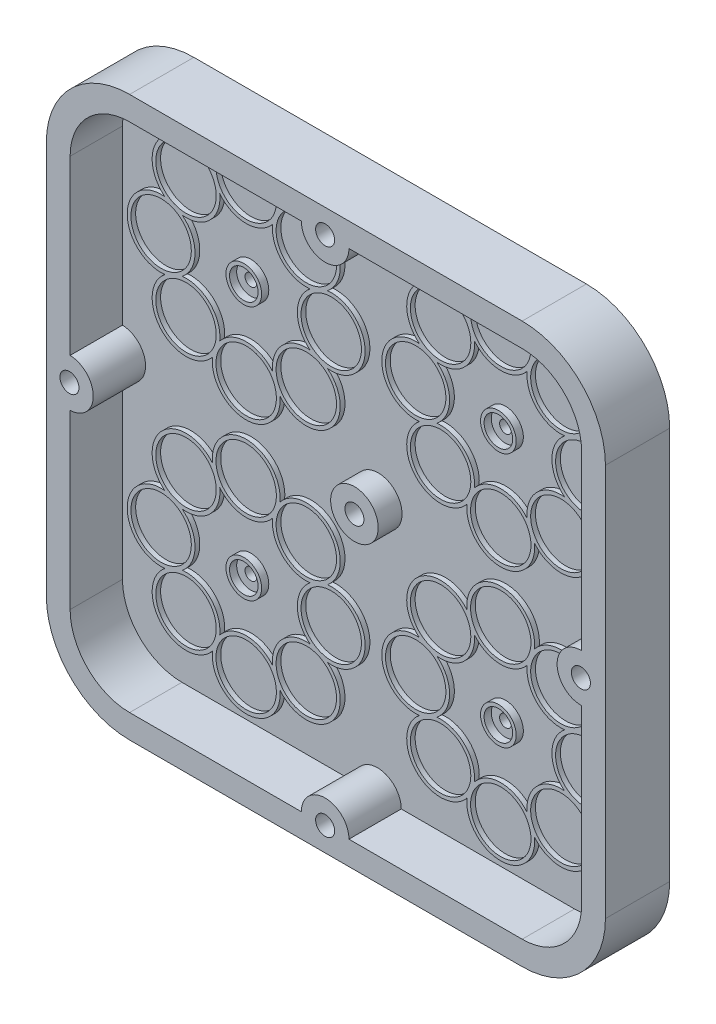
from build123d import *

# Parameters (mm, degrees)
SKETCH1_R           = 4
SKETCH1_R_2         = 2.5
BOSS_EXTRUDE1_DEPTH = 5
SKETCH2_R           = 4
BOSS_EXTRUDE2_DEPTH = 22
SKETCH3_R           = 10
SKETCH3_R_2         = 4
BOSS_EXTRUDE3_DEPTH = 10
SKETCH4_R           = 12.7
BOSS_EXTRUDE4_DEPTH = 2
SKETCH5_R           = 7.5
SKETCH5_R_2         = 6
BOSS_EXTRUDE5_DEPTH = 3


with BuildPart() as part:
    # Sketch1 → Boss-Extrude1 (new body)
    with BuildSketch(Plane.XY):
        with BuildLine():
            Line((35, 0), (200, 0))
            ThreePointArc((200, 0), (224.748737342, 10.251262658), (235, 35))
            Line((235, 35), (235, 200))
            ThreePointArc((235, 200), (224.748737342, 224.748737342), (200, 235))
            Line((200, 235), (35, 235))
            ThreePointArc((35, 235), (10.251262658, 224.748737342), (0, 200))
            Line((0, 200), (0, 35))
            ThreePointArc((0, 35), (10.251262658, 10.251262658), (35, 0))
        make_face()
        with Locations((117.5, 225)):
            Circle(SKETCH1_R, mode=Mode.SUBTRACT)
        with Locations((117.5, 10)):
            Circle(SKETCH1_R, mode=Mode.SUBTRACT)
        with Locations((117.5, 117.5)):
            Circle(SKETCH1_R, mode=Mode.SUBTRACT)
        with Locations((225, 117.5)):
            Circle(SKETCH1_R, mode=Mode.SUBTRACT)
        with Locations((10, 117.5)):
            Circle(SKETCH1_R, mode=Mode.SUBTRACT)
        with Locations((64, 171)):
            Circle(SKETCH1_R_2, mode=Mode.SUBTRACT)
        with Locations((171, 171)):
            Circle(SKETCH1_R_2, mode=Mode.SUBTRACT)
        with Locations((171, 64)):
            Circle(SKETCH1_R_2, mode=Mode.SUBTRACT)
        with Locations((64, 64)):
            Circle(SKETCH1_R_2, mode=Mode.SUBTRACT)
    extrude(amount=BOSS_EXTRUDE1_DEPTH)

    # Sketch2 → Boss-Extrude2 (add)
    with BuildSketch(Plane.XY.offset(5)):
        with BuildLine():
            Line((235, 35), (235, 200))
            ThreePointArc((235, 200), (224.748737342, 224.748737342), (200, 235))
            Line((200, 235), (35, 235))
            ThreePointArc((35, 235), (10.251262658, 224.748737342), (0, 200))
            Line((0, 200), (0, 35))
            ThreePointArc((0, 35), (10.251262658, 10.251262658), (35, 0))
            Line((35, 0), (200, 0))
            ThreePointArc((200, 0), (224.748737342, 10.251262658), (235, 35))
        make_face()
        with Locations(Location((117.185983795, 225.007361775, 0), (0, 0, 270.907179338))):
            Circle(SKETCH2_R, mode=Mode.SUBTRACT)
        with Locations(Location((224.685983795, 117.507361775, 0), (0, 0, 270.907179338))):
            Circle(SKETCH2_R, mode=Mode.SUBTRACT)
        with Locations(Location((117.185983795, 10.007361775, 0), (0, 0, 270.907179338))):
            Circle(SKETCH2_R, mode=Mode.SUBTRACT)
        with Locations(Location((9.72235037, 117.506509199, 0), (0, 0, 270.64647273))):
            Circle(SKETCH2_R, mode=Mode.SUBTRACT)
        with BuildLine():
            Line((200, 225), (127.185981085, 225))
            ThreePointArc((127.185981085, 225), (117.185983795, 215.007361775), (107.185986504, 225))
            Line((107.185986504, 225), (35, 225))
            ThreePointArc((35, 225), (17.32233047, 217.67766953), (10, 200))
            Line((10, 200), (10, 127.50265399))
            ThreePointArc((10, 127.50265399), (19.72235037, 117.506509199), (10, 107.510364408))
            Line((10, 107.510364408), (10, 35))
            ThreePointArc((10, 35), (17.32233047, 17.32233047), (35, 10))
            Line((35, 10), (107.185986504, 10))
            ThreePointArc((107.185986504, 10), (117.185983795, 20.007361775), (127.185981085, 10))
            Line((127.185981085, 10), (200, 10))
            ThreePointArc((200, 10), (217.67766953, 17.32233047), (225, 35))
            Line((225, 35), (225, 107.5122933))
            ThreePointArc((225, 107.5122933), (214.685983795, 117.507361775), (225, 127.50243025))
            Line((225, 127.50243025), (225, 200))
            ThreePointArc((225, 200), (217.67766953, 217.67766953), (200, 225))
        make_face(mode=Mode.SUBTRACT)
    extrude(amount=BOSS_EXTRUDE2_DEPTH)

    # Sketch3 → Boss-Extrude3 (add)
    with BuildSketch(Plane.XY.offset(5)):
        with Locations((117.5, 117.5)):
            Circle(SKETCH3_R)
        with Locations((117.5, 117.5)):
            Circle(SKETCH3_R_2, mode=Mode.SUBTRACT)
    extrude(amount=BOSS_EXTRUDE3_DEPTH)

    # Sketch4 → Boss-Extrude4 (add)
    # profile 1 of 4: a face of its own
    with BuildSketch(Plane.XY.offset(5)):
        with BuildLine():
            ThreePointArc((136.802142668, 185.165216311), (121, 171), (136.802142668, 156.834783689))
            ThreePointArc((136.802142668, 156.834783689), (135.644660941, 135.644660941), (156.834783689, 136.802142668))
            ThreePointArc((156.834783689, 136.802142668), (171, 121), (185.165216311, 136.802142668))
            ThreePointArc((185.165216311, 136.802142668), (206.355339059, 135.644660941), (205.197857332, 156.834783689))
            ThreePointArc((205.197857332, 156.834783689), (221, 171), (205.197857332, 185.165216311))
            ThreePointArc((205.197857332, 185.165216311), (206.355339059, 206.355339059), (185.165216311, 205.197857332))
            ThreePointArc((185.165216311, 205.197857332), (171, 221), (156.834783689, 205.197857332))
            ThreePointArc((156.834783689, 205.197857332), (135.644660941, 206.355339059), (136.802142668, 185.165216311))
        make_face()
        with Locations((171, 206.75)):
            Circle(SKETCH4_R, mode=Mode.SUBTRACT)
        with Locations((145.720932573, 196.279067427)):
            Circle(SKETCH4_R, mode=Mode.SUBTRACT)
        with Locations((135.25, 171)):
            Circle(SKETCH4_R, mode=Mode.SUBTRACT)
        with Locations((145.720932573, 145.720932573)):
            Circle(SKETCH4_R, mode=Mode.SUBTRACT)
        with Locations((171, 135.25)):
            Circle(SKETCH4_R, mode=Mode.SUBTRACT)
        with Locations((196.279067427, 145.720932573)):
            Circle(SKETCH4_R, mode=Mode.SUBTRACT)
        with Locations((206.75, 171)):
            Circle(SKETCH4_R, mode=Mode.SUBTRACT)
        with Locations((196.279067427, 196.279067427)):
            Circle(SKETCH4_R, mode=Mode.SUBTRACT)
        with BuildLine():
            ThreePointArc((159.886148884, 197.831210095), (171, 192.5), (182.113851116, 197.831210095))
            ThreePointArc((182.113851116, 197.831210095), (186.202795796, 186.202795796), (197.831210095, 182.113851116))
            ThreePointArc((197.831210095, 182.113851116), (192.5, 171), (197.831210095, 159.886148884))
            ThreePointArc((197.831210095, 159.886148884), (186.202795796, 155.797204204), (182.113851116, 144.168789905))
            ThreePointArc((182.113851116, 144.168789905), (171, 149.5), (159.886148884, 144.168789905))
            ThreePointArc((159.886148884, 144.168789905), (155.797204204, 155.797204204), (144.168789905, 159.886148884))
            ThreePointArc((144.168789905, 159.886148884), (149.5, 171), (144.168789905, 182.113851116))
            ThreePointArc((144.168789905, 182.113851116), (155.797204204, 186.202795796), (159.886148884, 197.831210095))
        make_face(mode=Mode.SUBTRACT)
    # profile 2 of 4: a face of its own
    with BuildSketch(Plane.XY.offset(5)):
        with BuildLine():
            ThreePointArc((185.165216311, 98.197857332), (171, 114), (156.834783689, 98.197857332))
            ThreePointArc((156.834783689, 98.197857332), (135.644660941, 99.355339059), (136.802142668, 78.165216311))
            ThreePointArc((136.802142668, 78.165216311), (121, 64), (136.802142668, 49.834783689))
            ThreePointArc((136.802142668, 49.834783689), (135.644660941, 28.644660941), (156.834783689, 29.802142668))
            ThreePointArc((156.834783689, 29.802142668), (171, 14), (185.165216311, 29.802142668))
            ThreePointArc((185.165216311, 29.802142668), (206.355339059, 28.644660941), (205.197857332, 49.834783689))
            ThreePointArc((205.197857332, 49.834783689), (221, 64), (205.197857332, 78.165216311))
            ThreePointArc((205.197857332, 78.165216311), (206.355339059, 99.355339059), (185.165216311, 98.197857332))
        make_face()
        with Locations((171, 99.75)):
            Circle(SKETCH4_R, mode=Mode.SUBTRACT)
        with Locations((145.720932573, 89.279067427)):
            Circle(SKETCH4_R, mode=Mode.SUBTRACT)
        with Locations((135.25, 64)):
            Circle(SKETCH4_R, mode=Mode.SUBTRACT)
        with Locations((145.720932573, 38.720932573)):
            Circle(SKETCH4_R, mode=Mode.SUBTRACT)
        with Locations((171, 28.25)):
            Circle(SKETCH4_R, mode=Mode.SUBTRACT)
        with Locations((196.279067427, 38.720932573)):
            Circle(SKETCH4_R, mode=Mode.SUBTRACT)
        with Locations((206.75, 64)):
            Circle(SKETCH4_R, mode=Mode.SUBTRACT)
        with Locations((196.279067427, 89.279067427)):
            Circle(SKETCH4_R, mode=Mode.SUBTRACT)
        with BuildLine():
            ThreePointArc((144.168789905, 75.113851116), (155.797204204, 79.202795796), (159.886148884, 90.831210095))
            ThreePointArc((159.886148884, 90.831210095), (171, 85.5), (182.113851116, 90.831210095))
            ThreePointArc((182.113851116, 90.831210095), (186.202795796, 79.202795796), (197.831210095, 75.113851116))
            ThreePointArc((197.831210095, 75.113851116), (192.5, 64), (197.831210095, 52.886148884))
            ThreePointArc((197.831210095, 52.886148884), (186.202795796, 48.797204204), (182.113851116, 37.168789905))
            ThreePointArc((182.113851116, 37.168789905), (171, 42.5), (159.886148884, 37.168789905))
            ThreePointArc((159.886148884, 37.168789905), (155.797204204, 48.797204204), (144.168789905, 52.886148884))
            ThreePointArc((144.168789905, 52.886148884), (149.5, 64), (144.168789905, 75.113851116))
        make_face(mode=Mode.SUBTRACT)
    # profile 3 of 4: a face of its own
    with BuildSketch(Plane.XY.offset(5)):
        with BuildLine():
            ThreePointArc((98.197857332, 49.834783689), (114, 64), (98.197857332, 78.165216311))
            ThreePointArc((98.197857332, 78.165216311), (99.355339059, 99.355339059), (78.165216311, 98.197857332))
            ThreePointArc((78.165216311, 98.197857332), (64, 114), (49.834783689, 98.197857332))
            ThreePointArc((49.834783689, 98.197857332), (28.644660941, 99.355339059), (29.802142668, 78.165216311))
            ThreePointArc((29.802142668, 78.165216311), (14, 64), (29.802142668, 49.834783689))
            ThreePointArc((29.802142668, 49.834783689), (28.644660941, 28.644660941), (49.834783689, 29.802142668))
            ThreePointArc((49.834783689, 29.802142668), (64, 14), (78.165216311, 29.802142668))
            ThreePointArc((78.165216311, 29.802142668), (99.355339059, 28.644660941), (98.197857332, 49.834783689))
        make_face()
        with Locations((99.75, 64)):
            Circle(SKETCH4_R, mode=Mode.SUBTRACT)
        with Locations((89.279067427, 89.279067427)):
            Circle(SKETCH4_R, mode=Mode.SUBTRACT)
        with Locations((64, 99.75)):
            Circle(SKETCH4_R, mode=Mode.SUBTRACT)
        with Locations((38.720932573, 89.279067427)):
            Circle(SKETCH4_R, mode=Mode.SUBTRACT)
        with Locations((28.25, 64)):
            Circle(SKETCH4_R, mode=Mode.SUBTRACT)
        with Locations((38.720932573, 38.720932573)):
            Circle(SKETCH4_R, mode=Mode.SUBTRACT)
        with Locations((64, 28.25)):
            Circle(SKETCH4_R, mode=Mode.SUBTRACT)
        with Locations((89.279067427, 38.720932573)):
            Circle(SKETCH4_R, mode=Mode.SUBTRACT)
        with BuildLine():
            ThreePointArc((75.113851116, 90.831210095), (79.202795796, 79.202795796), (90.831210095, 75.113851116))
            ThreePointArc((90.831210095, 75.113851116), (85.5, 64), (90.831210095, 52.886148884))
            ThreePointArc((90.831210095, 52.886148884), (79.202795796, 48.797204204), (75.113851116, 37.168789905))
            ThreePointArc((75.113851116, 37.168789905), (64, 42.5), (52.886148884, 37.168789905))
            ThreePointArc((52.886148884, 37.168789905), (48.797204204, 48.797204204), (37.168789905, 52.886148884))
            ThreePointArc((37.168789905, 52.886148884), (42.5, 64), (37.168789905, 75.113851116))
            ThreePointArc((37.168789905, 75.113851116), (48.797204204, 79.202795796), (52.886148884, 90.831210095))
            ThreePointArc((52.886148884, 90.831210095), (64, 85.5), (75.113851116, 90.831210095))
        make_face(mode=Mode.SUBTRACT)
    # profile 4 of 4: a face of its own
    with BuildSketch(Plane.XY.offset(5)):
        with BuildLine():
            ThreePointArc((49.834783689, 136.802142668), (64, 121), (78.165216311, 136.802142668))
            ThreePointArc((78.165216311, 136.802142668), (99.355339059, 135.644660941), (98.197857332, 156.834783689))
            ThreePointArc((98.197857332, 156.834783689), (114, 171), (98.197857332, 185.165216311))
            ThreePointArc((98.197857332, 185.165216311), (99.355339059, 206.355339059), (78.165216311, 205.197857332))
            ThreePointArc((78.165216311, 205.197857332), (64, 221), (49.834783689, 205.197857332))
            ThreePointArc((49.834783689, 205.197857332), (28.644660941, 206.355339059), (29.802142668, 185.165216311))
            ThreePointArc((29.802142668, 185.165216311), (14, 171), (29.802142668, 156.834783689))
            ThreePointArc((29.802142668, 156.834783689), (28.644660941, 135.644660941), (49.834783689, 136.802142668))
        make_face()
        with Locations((64, 135.25)):
            Circle(SKETCH4_R, mode=Mode.SUBTRACT)
        with Locations((89.279067427, 145.720932573)):
            Circle(SKETCH4_R, mode=Mode.SUBTRACT)
        with Locations((99.75, 171)):
            Circle(SKETCH4_R, mode=Mode.SUBTRACT)
        with Locations((89.279067427, 196.279067427)):
            Circle(SKETCH4_R, mode=Mode.SUBTRACT)
        with Locations((64, 206.75)):
            Circle(SKETCH4_R, mode=Mode.SUBTRACT)
        with Locations((38.720932573, 196.279067427)):
            Circle(SKETCH4_R, mode=Mode.SUBTRACT)
        with Locations((28.25, 171)):
            Circle(SKETCH4_R, mode=Mode.SUBTRACT)
        with Locations((38.720932573, 145.720932573)):
            Circle(SKETCH4_R, mode=Mode.SUBTRACT)
        with BuildLine():
            ThreePointArc((90.831210095, 159.886148884), (79.202795796, 155.797204204), (75.113851116, 144.168789905))
            ThreePointArc((75.113851116, 144.168789905), (64, 149.5), (52.886148884, 144.168789905))
            ThreePointArc((52.886148884, 144.168789905), (48.797204204, 155.797204204), (37.168789905, 159.886148884))
            ThreePointArc((37.168789905, 159.886148884), (42.5, 171), (37.168789905, 182.113851116))
            ThreePointArc((37.168789905, 182.113851116), (48.797204204, 186.202795796), (52.886148884, 197.831210095))
            ThreePointArc((52.886148884, 197.831210095), (64, 192.5), (75.113851116, 197.831210095))
            ThreePointArc((75.113851116, 197.831210095), (79.202795796, 186.202795796), (90.831210095, 182.113851116))
            ThreePointArc((90.831210095, 182.113851116), (85.5, 171), (90.831210095, 159.886148884))
        make_face(mode=Mode.SUBTRACT)
    extrude(amount=BOSS_EXTRUDE4_DEPTH)

    # Sketch5 → Boss-Extrude5 (add)
    # profile 1 of 4: a face of its own
    with BuildSketch(Plane.XY.offset(5)):
        with Locations((171, 171)):
            Circle(SKETCH5_R)
        with Locations((171, 171)):
            Circle(SKETCH5_R_2, mode=Mode.SUBTRACT)
    # profile 2 of 4: a face of its own
    with BuildSketch(Plane.XY.offset(5)):
        with Locations((64, 171)):
            Circle(SKETCH5_R)
        with Locations((64, 171)):
            Circle(SKETCH5_R_2, mode=Mode.SUBTRACT)
    # profile 3 of 4: a face of its own
    with BuildSketch(Plane.XY.offset(5)):
        with Locations((64, 64)):
            Circle(SKETCH5_R)
        with Locations((64, 64)):
            Circle(SKETCH5_R_2, mode=Mode.SUBTRACT)
    # profile 4 of 4: a face of its own
    with BuildSketch(Plane.XY.offset(5)):
        with Locations((171, 64)):
            Circle(SKETCH5_R)
        with Locations((171, 64)):
            Circle(SKETCH5_R_2, mode=Mode.SUBTRACT)
    extrude(amount=BOSS_EXTRUDE5_DEPTH)


solid = part.part
